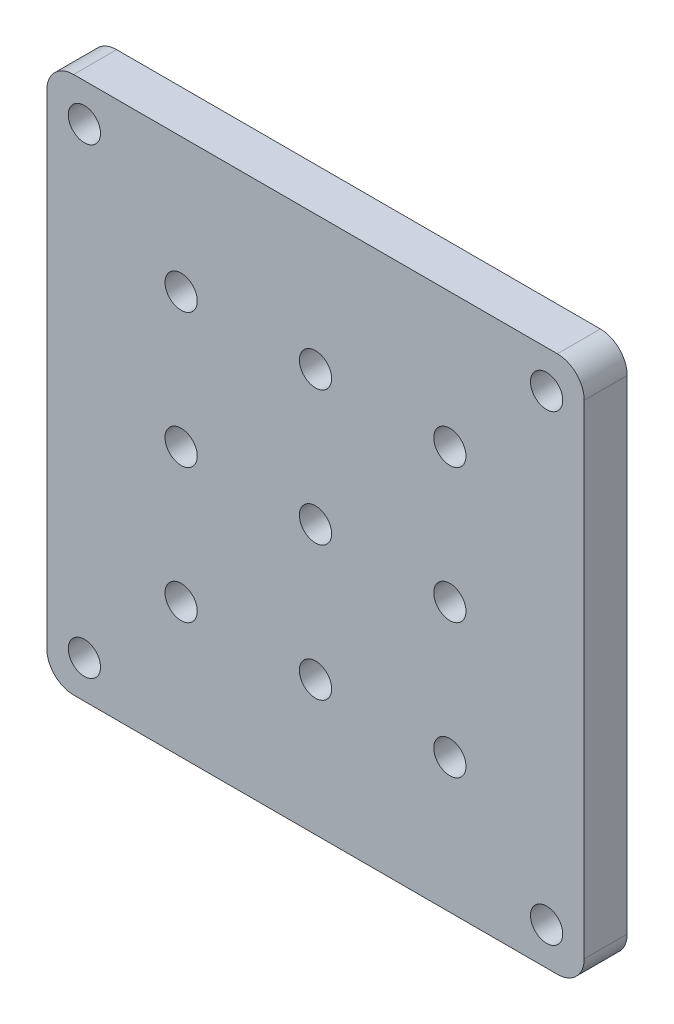
SolidWorks part; units mm, degrees
ref_plane "Front Plane" through (0, 0, 0) normal (0, 0, 1) x (1, 0, 0)
ref_plane "Top Plane" through (0, 0, 0) normal (0, 1, 0) x (1, 0, 0)
ref_plane "Right Plane" through (0, 0, 0) normal (1, 0, 0) x (0, 0, -1)
other "Configuration Table"
sketch "Sketch1" plane through (0, 0, 0) normal (0, 0, 1) x (1, 0, 0)
  line L0 (-25, 50) -> (-25, -50) construction
  line L1 (-45, 50) -> (45, 50)
  line L2 (-50, 45) -> (-50, -45)
  line L3 (-45, -50) -> (45, -50)
  line L4 (50, 45) -> (50, -45)
  line L5 (-50, 50) -> (50, -50) construction
  line L6 (-50, -50) -> (50, 50) construction
  line L7 (0, 50) -> (0, -50) construction
  line L8 (-50, 25) -> (50, 25) construction
  line L10 (-43, 43) -> (43, 43) construction
  line L11 (-43, 43) -> (-43, -43) construction
  line L12 (-43, -43) -> (43, -43) construction
  line L13 (43, 43) -> (43, -43) construction
  line L14 (-43, 43) -> (43, -43) construction
  line L15 (-43, -43) -> (43, 43) construction
  arc A0 (45, -50) -> (50, -45) centre (45, -45) ccw
  arc A1 (-50, -45) -> (-45, -50) centre (-45, -45) ccw
  arc A2 (45, 50) -> (50, 45) centre (45, 45) cw
  arc A3 (-45, 50) -> (-50, 45) centre (-45, 45) ccw
  circle A4 centre (-25, 25) radius 3
  circle A5 centre (0, 25) radius 3
  circle A6 centre (25, 25) radius 3
  circle A7 centre (0, 0) radius 3
  circle A8 centre (25, 0) radius 3
  circle A9 centre (0, -25) radius 3
  circle A10 centre (25, -25) radius 3
  circle A11 centre (-25, 0) radius 3
  circle A12 centre (-25, -25) radius 3
  circle A14 centre (43, 43) radius 3
  circle A15 centre (43, -43) radius 3
  circle A16 centre (-43, -43) radius 3
  circle A17 centre (-43, 43) radius 3
  point P0 (0, 0)
  dimension "D3" = 5
  dimension "D6" = 6
  dimension "D10" = 6
  dimension "D1" = 100
  dimension "D2" = 100
  dimension "D4" = 25
  dimension "D5" = 25
  dimension "D9" = 86
  dimension "D7" = 3
  dimension "D8" = 3
extrude "Boss-Extrude1" add sketch "Sketch1" along normal blind 8
